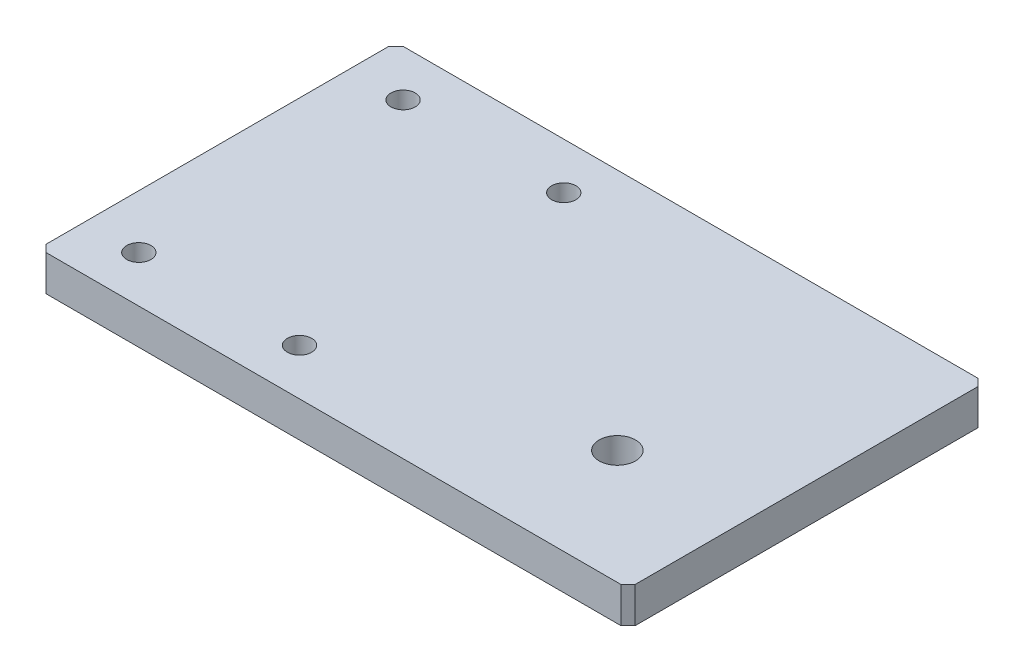
from build123d import *

# Parameters (mm, degrees)
SKETCH_1_W              = 165
SKETCH_1_H              = 100
EXTRUDE_1_DEPTH         = 10
HOLE_WIZARD_M8_1_D      = 6.8
HOLE_WIZARD_M8_1_DEPTH  = 16.25
HOLE_WIZARD_M8_1_TIP    = 2.042926105
HOLE_WIZARD_M12_1_D     = 10.2
HOLE_WIZARD_M12_1_DEPTH = 32.75
HOLE_WIZARD_M12_1_TIP   = 3.064389157
CHAMFER_1_SIZE          = 2


with BuildPart() as part:
    # 草图1 → 凸台-拉伸1 (new body)
    with BuildSketch(Plane(origin=(0, 0, 0), x_dir=(1, 0, 0), z_dir=(0, 1, 0))):
        Rectangle(SKETCH_1_W, SKETCH_1_H)
    extrude(amount=EXTRUDE_1_DEPTH)

    # M8 螺纹孔1
    with Locations(Plane(origin=(0, 10, 0), x_dir=(1, 0, 0), z_dir=(0, 1, 0))):
        with Locations((-67.5, 37), (-22.5, 37), (-22.5, -37), (-67.5, -37)):
            Hole(HOLE_WIZARD_M8_1_D / 2, depth=HOLE_WIZARD_M8_1_DEPTH)
            with Locations((0, 0, -(HOLE_WIZARD_M8_1_DEPTH + HOLE_WIZARD_M8_1_TIP / 2))):  # 118° drill point
                Cone(0, HOLE_WIZARD_M8_1_D / 2, HOLE_WIZARD_M8_1_TIP, mode=Mode.SUBTRACT)

    # M12 螺纹孔1
    with Locations(Plane(origin=(0, 10, 0), x_dir=(1, 0, 0), z_dir=(0, 1, 0))):
        with Locations((47.5, -18)):
            Hole(HOLE_WIZARD_M12_1_D / 2, depth=HOLE_WIZARD_M12_1_DEPTH)
            with Locations((0, 0, -(HOLE_WIZARD_M12_1_DEPTH + HOLE_WIZARD_M12_1_TIP / 2))):  # 118° drill point
                Cone(0, HOLE_WIZARD_M12_1_D / 2, HOLE_WIZARD_M12_1_TIP, mode=Mode.SUBTRACT)

    # 倒角1
    chamfer_1_edges = [part.edges().sort_by_distance(p)[0] for p in [
        (82.5, 5, 50),
        (-82.5, 5, 50),
        (-82.5, 5, -50),
        (82.5, 5, -50),
    ]]
    chamfer(chamfer_1_edges, length=CHAMFER_1_SIZE)


solid = part.part
